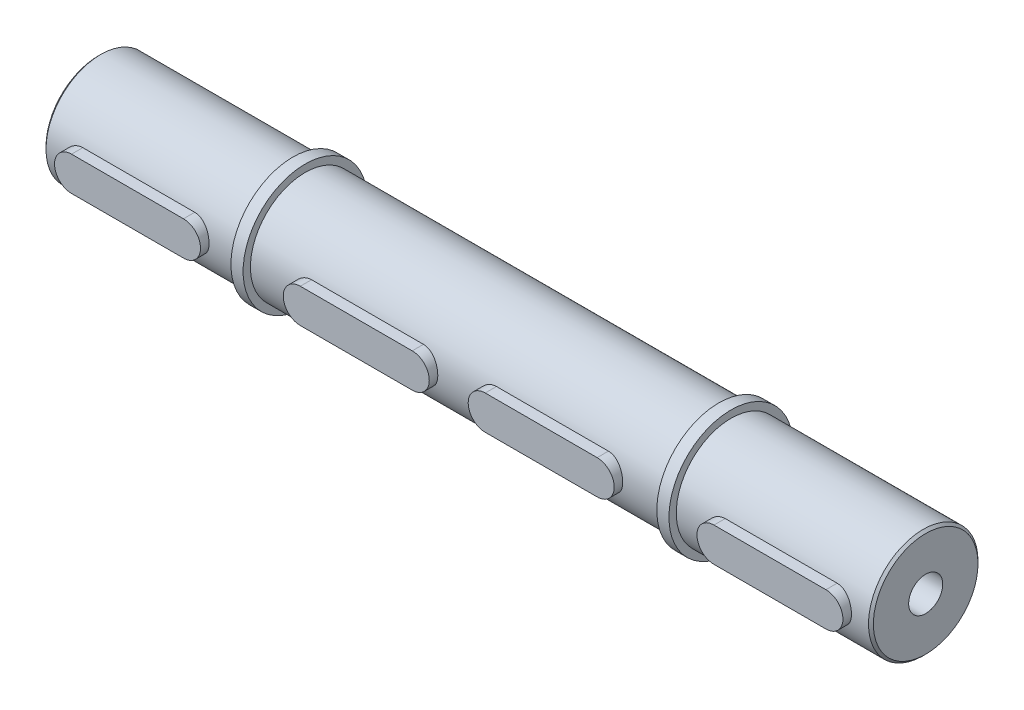
from build123d import *

# Parameters (mm, degrees)
CHAMFER1_SIZE        = 1
BOSS_EXTRUDE1_DEPTH  = 26
MIRROR6_COPY_1_DEPTH = 26


with BuildPart() as part:
    # Sketch1 → Revolve1 (revolve)
    with BuildSketch(Plane.XY, mode=Mode.PRIVATE) as revolve1_sk:
        Polygon((170, 0), (-170, 0), (-170, 22.5), (-90, 22.5), (-90, 25.5), (-85, 25.5), (-85, 22.5), (85, 22.5), (85, 25.5), (90, 25.5), (90, 22.5), (170, 22.5), align=None)
    revolve(revolve1_sk.sketch.rotate(Axis((170, 0, 0), (-1, 0, 0)), 90), axis=Axis((170, 0, 0), (-1, 0, 0)))

    # Chamfer1
    chamfer1_edges = [part.edges().sort_by_distance(p)[0] for p in [
        (-170, 0, 22.5),
        (170, 0, 22.5),
    ]]
    chamfer(chamfer1_edges, length=CHAMFER1_SIZE)

    # Sketch2 → Boss-Extrude1 (add)
    with BuildSketch(Plane.XY):
        with BuildLine():
            Line((-155, 7), (-109, 7))
            ThreePointArc((-109, 7), (-102, 0), (-109, -7))
            Line((-109, -7), (-155, -7))
            ThreePointArc((-155, -7), (-162, 0), (-155, 7))
        make_face()
    boss_extrude1 = extrude(amount=BOSS_EXTRUDE1_DEPTH)

    # Mirror1: Boss-Extrude1 across plane
    add(boss_extrude1.mirror(Plane(origin=(0, 0, 0), x_dir=(0, 0, 1), z_dir=(1, 0, 0))))

    # Sketch3 → M16 Tapped Hole1 (revolve, cut)
    with BuildSketch(Plane(origin=(-170, 0, 0), x_dir=(0, 0, 1), z_dir=(0, 1, 0))):
        Polygon((0, 0), (0, 22.206024333), (7, 18), (7, 0), align=None)
    m16_tapped_hole1 = revolve(axis=Axis((-176.35, 0, 0), (1, 0, 0)), mode=Mode.SUBTRACT)

    # Mirror2: M16 Tapped Hole1 across plane
    add(m16_tapped_hole1.mirror(Plane(origin=(0, 0, 0), x_dir=(0, 0, 1), z_dir=(1, 0, 0))), mode=Mode.SUBTRACT)

    # Mirror3: Boss-Extrude1 across plane
    add(boss_extrude1.mirror(Plane(origin=(-85, 25.5, 0), x_dir=(0, 0, 1), z_dir=(1, 0, 0))))

    # Mirror6 copy 1 sketch → Mirror6 copy 1 (add)
    with BuildSketch(Plane(origin=(170, 0, 0), x_dir=(1, 0, 0), z_dir=(0, 0, 1))):
        with BuildLine():
            Line((-155, 7), (-109, 7))
            ThreePointArc((-109, 7), (-102, 0), (-109, -7))
            Line((-109, -7), (-155, -7))
            ThreePointArc((-155, -7), (-162, 0), (-155, 7))
        make_face()
    extrude(amount=MIRROR6_COPY_1_DEPTH)


solid = part.part
